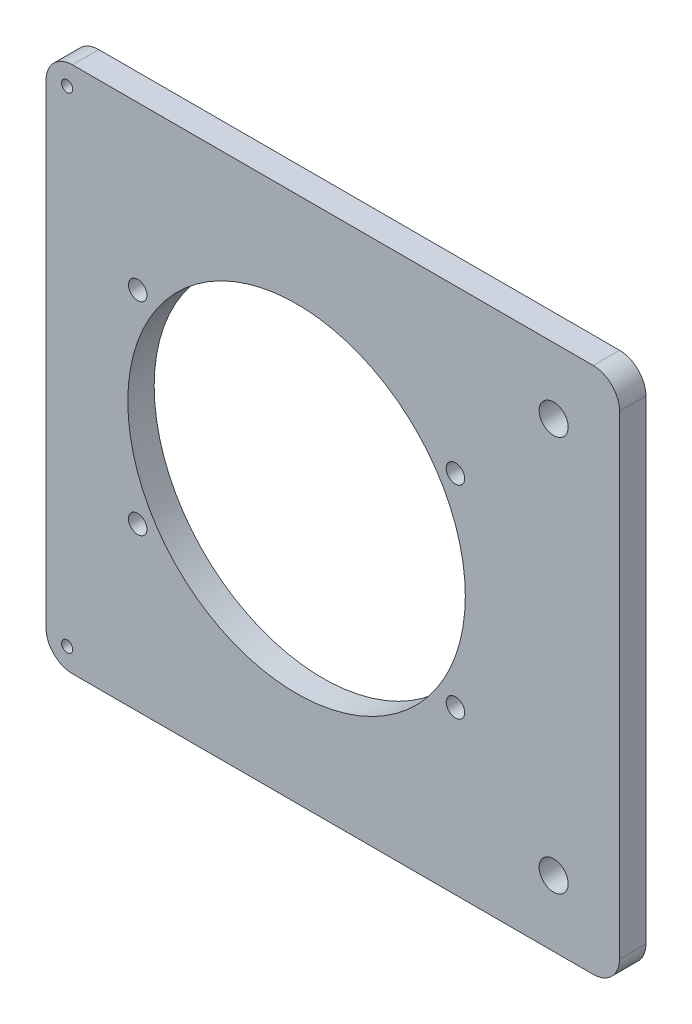
from build123d import *

# Parameters (mm, degrees)
SKETCH1_W             = 190
SKETCH1_H             = 200
BOSS_EXTRUDE1_DEPTH   = 10
SKETCH2_R             = 64
CUT_EXTRUDE1_DEPTH    = 10
SKETCH3_R             = 3.5
CUT_EXTRUDE2_DEPTH    = 10
SKETCH4_W             = 27.5
SKETCH4_H             = 200
BOSS_EXTRUDE2_DEPTH   = 10
SKETCH5_R             = 5.5
CUT_EXTRUDE3_DEPTH    = 10
SKETCH6_R             = 0.5
CUT_EXTRUDE4_DEPTH    = 10
M5_TAPPED_HOLE1_D     = 4.2
M5_TAPPED_HOLE1_DEPTH = 14
M5_TAPPED_HOLE1_TIP   = 1.2618073
FILLET1_R             = 10


with BuildPart() as part:
    # Sketch1 → Boss-Extrude1 (new body)
    with BuildSketch(Plane.XY):
        Rectangle(SKETCH1_W, SKETCH1_H)
    extrude(amount=BOSS_EXTRUDE1_DEPTH)

    # Sketch2 → Cut-Extrude1 (cut)
    with BuildSketch(Plane.XY.offset(10)):
        Circle(SKETCH2_R)
    extrude(amount=-CUT_EXTRUDE1_DEPTH, mode=Mode.SUBTRACT)

    # Sketch3 → Cut-Extrude2 (cut)
    with BuildSketch(Plane.XY.offset(10)):
        with Locations((-60.25, 38.425)):
            Circle(SKETCH3_R)
        with Locations(Location((60.25, 38.425, 0), (0, 0, 180))):
            Circle(SKETCH3_R)
        with Locations((60.25, -38.425)):
            Circle(SKETCH3_R)
        with Locations(Location((-60.25, -38.425, 0), (0, 0, 180))):
            Circle(SKETCH3_R)
    extrude(amount=-CUT_EXTRUDE2_DEPTH, mode=Mode.SUBTRACT)

    # Sketch4 → Boss-Extrude2 (add)
    with BuildSketch(Plane.XY.offset(10)):
        with Locations((108.75, 0)):
            Rectangle(SKETCH4_W, SKETCH4_H)
    extrude(amount=-BOSS_EXTRUDE2_DEPTH)

    # Sketch5 → Cut-Extrude3 (cut)
    with BuildSketch(Plane.XY.offset(10)):
        with Locations((97.5, 75)):
            Circle(SKETCH5_R)
        with Locations(Location((97.5, -75, 0), (0, 0, 180))):
            Circle(SKETCH5_R)
    extrude(amount=-CUT_EXTRUDE3_DEPTH, mode=Mode.SUBTRACT)

    # Sketch6 → Cut-Extrude4 (cut)
    with BuildSketch(Plane.XY.offset(10)):
        with Locations((-87, -92)):
            Circle(SKETCH6_R)
        with Locations(Location((-87, 92, 0), (0, 0, 180))):
            Circle(SKETCH6_R)
    extrude(amount=-CUT_EXTRUDE4_DEPTH, mode=Mode.SUBTRACT)

    # M5 Tapped Hole1
    with Locations(Plane.XY.offset(10)):
        with Locations((-87, 92), (-87, -92)):
            Hole(M5_TAPPED_HOLE1_D / 2, depth=M5_TAPPED_HOLE1_DEPTH)
            with Locations((0, 0, -(M5_TAPPED_HOLE1_DEPTH + M5_TAPPED_HOLE1_TIP / 2))):  # 118° drill point
                Cone(0, M5_TAPPED_HOLE1_D / 2, M5_TAPPED_HOLE1_TIP, mode=Mode.SUBTRACT)

    # Fillet1
    fillet1_edges = [part.edges().sort_by_distance(p)[0] for p in [
        (122.5, 100, 5),
        (122.5, -100, 5),
        (-95, -100, 5),
        (-95, 100, 5),
    ]]
    fillet(fillet1_edges, radius=FILLET1_R)


solid = part.part
